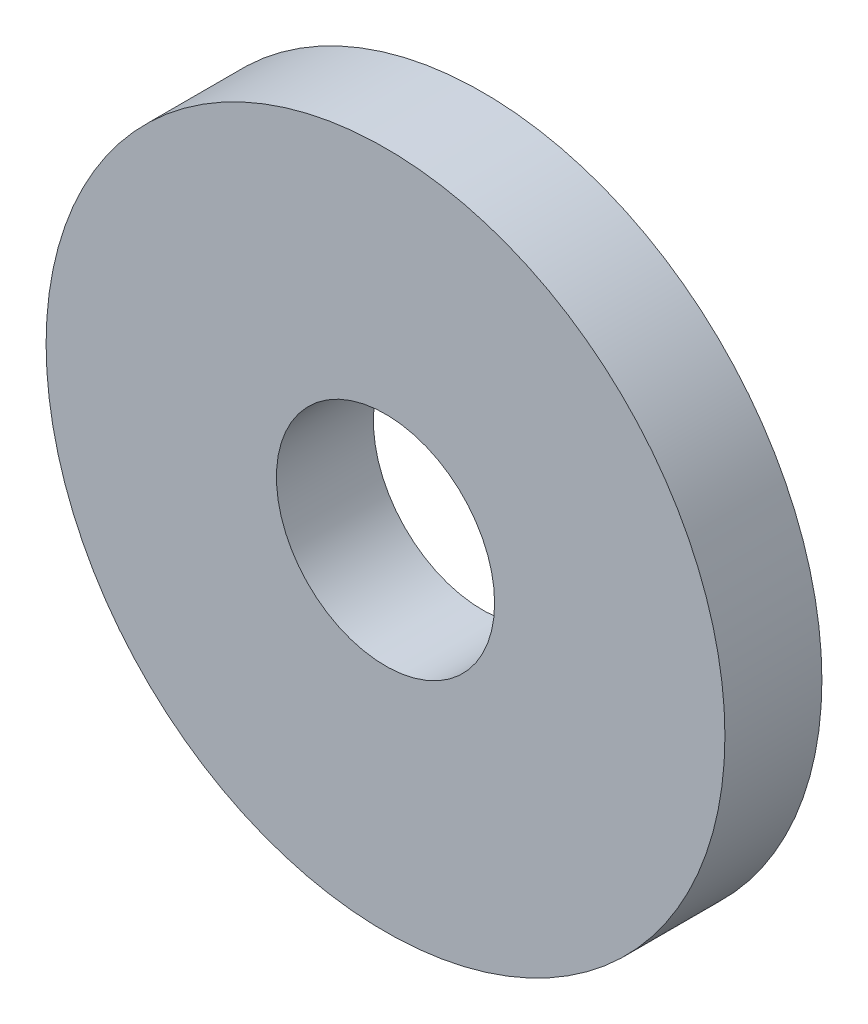
SolidWorks part; units mm, degrees
material "S45C"
ref_plane "Front Plane" through (0, 0, 0) normal (0, 0, 1) x (1, 0, 0)
ref_plane "Top Plane" through (0, 0, 0) normal (0, 1, 0) x (1, 0, 0)
ref_plane "Right Plane" through (0, 0, 0) normal (1, 0, 0) x (0, 0, -1)
sketch "Sketch1" plane through (0, 0, 0) normal (0, 0, 1) x (1, 0, 0)
  circle A0 centre (0, 0) radius 2.25
  circle A1 centre (0, 0) radius 7
  dimension "D1" = 4.5
  dimension "D2" = 14
extrude "Boss-Extrude1" add sketch "Sketch1" along normal blind 2
